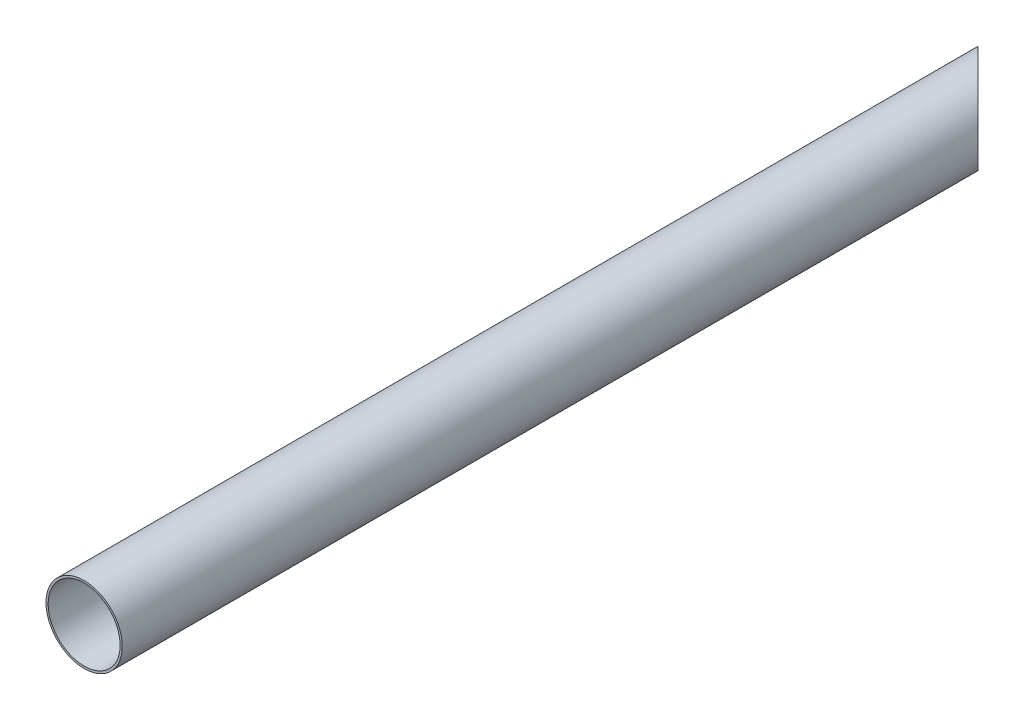
SolidWorks part; units mm, degrees
ref_plane "Front Plane" through (0, 0, 0) normal (0, 0, 1) x (1, 0, 0)
ref_plane "Top Plane" through (0, 0, 0) normal (0, 1, 0) x (1, 0, 0)
ref_plane "Right Plane" through (0, 0, 0) normal (1, 0, 0) x (0, 0, -1)
sketch "Sketch1" plane through (0, 0, 0) normal (0, 0, 1) x (1, 0, 0)
  circle A0 centre (0, 0) radius 8.5
  circle A1 centre (0, 0) radius 9
extrude "Boss-Extrude1" add sketch "Sketch1" along normal blind 220
sketch "Sketch2" plane through (0, 0, 0) normal (0, 1, 0) x (1, 0, 0)
  line L0 (-9, 0) -> (9, 0)
  line L1 (-9, 0) -> (9, -18)
  line L2 (9, -18) -> (9, 0)
  line L3 (9, -220) -> (9, 0) construction
  dimension "D1" = 45
extrude "Cut-Extrude1" cut sketch "Sketch2" against normal mid plane 220
